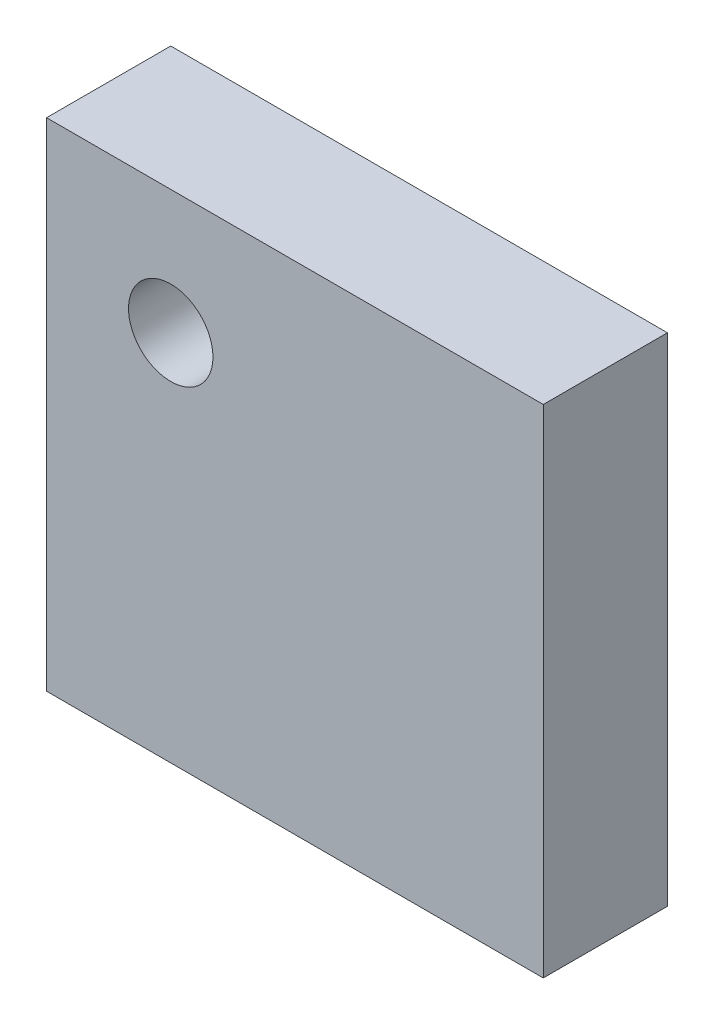
from build123d import *

# Parameters (mm, degrees)
SKETCH_1_W         = 40
SKETCH_1_H         = 40
EXTRUDE_1_DEPTH    = 5
HOLE_WIZARD_M8_1_D = 6.8


with BuildPart() as part:
    # 草图1 → 凸台-拉伸1 (new, symmetric)
    with BuildSketch(Plane.XY):
        Rectangle(SKETCH_1_W, SKETCH_1_H)
    extrude(amount=EXTRUDE_1_DEPTH, both=True)

    # M8 螺纹孔1 (through all)
    with Locations(Plane.XY.offset(5)):
        with Locations((-10, 10)):
            Hole(HOLE_WIZARD_M8_1_D / 2)


solid = part.part
